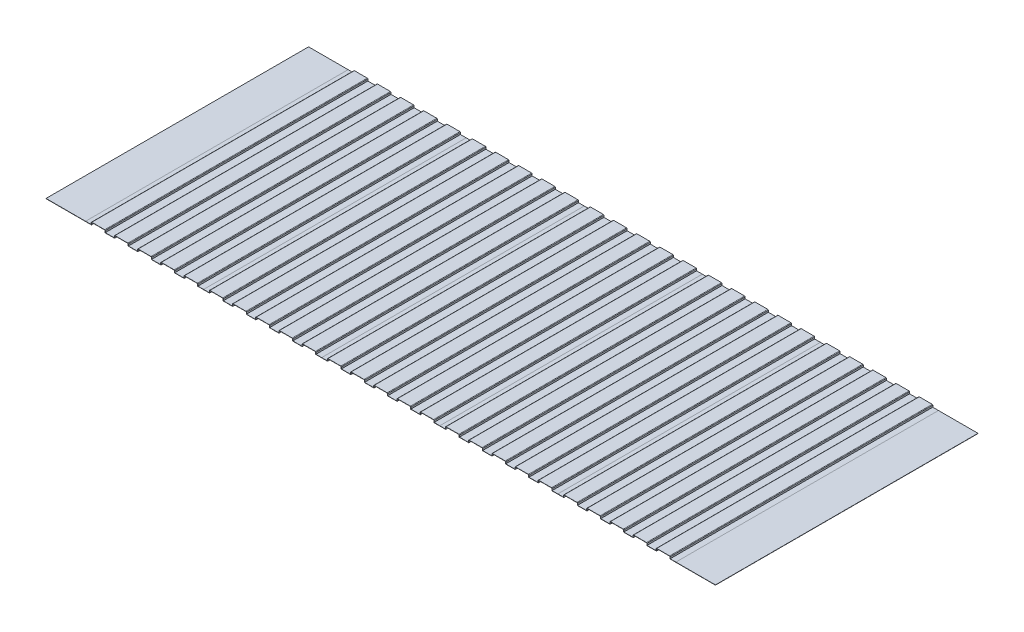
SolidWorks part; units mm, degrees
ref_plane "Front Plane" through (0, 0, 0) normal (0, 0, 1) x (1, 0, 0)
ref_plane "Top Plane" through (0, 0, 0) normal (0, 1, 0) x (1, 0, 0)
ref_plane "Right Plane" through (0, 0, 0) normal (1, 0, 0) x (0, 0, -1)
other "Configuration Table"
sketch "Sketch1" plane through (0, 0, 0) normal (0, 0, 1) x (1, 0, 0)
  line L0 (1045, 2) -> (994.5, 2)
  line L1 (994.5, 2) -> (994.5, 17)
  line L2 (989.5, 22) -> (875.5, 22)
  line L3 (870.5, 17) -> (870.5, 2)
  line L4 (870.5, 2) -> (789.5, 2)
  line L5 (789.5, 2) -> (789.5, 17)
  line L6 (784.5, 22) -> (670.5, 22)
  line L7 (665.5, 17) -> (665.5, 2)
  line L8 (665.5, 2) -> (584.5, 2)
  line L9 (584.5, 2) -> (584.5, 17)
  line L10 (579.5, 22) -> (465.5, 22)
  line L11 (460.5, 17) -> (460.5, 2)
  line L12 (460.5, 2) -> (379.5, 2)
  line L13 (379.5, 2) -> (379.5, 17)
  line L14 (374.5, 22) -> (260.5, 22)
  line L15 (255.5, 17) -> (255.5, 2)
  line L16 (255.5, 2) -> (174.5, 2)
  line L17 (174.5, 2) -> (174.5, 17)
  line L18 (169.5, 22) -> (55.5, 22)
  line L19 (50.5, 17) -> (50.5, 2)
  line L20 (50.5, 2) -> (0, 2)
  line L21 (0, 2) -> (0, 0)
  line L22 (0, 0) -> (52.5, 0)
  line L23 (52.5, 0) -> (52.5, 17)
  line L24 (55.5, 20) -> (169.5, 20)
  line L25 (172.5, 17) -> (172.5, 0)
  line L26 (172.5, 0) -> (257.5, 0)
  line L27 (257.5, 0) -> (257.5, 17)
  line L28 (260.5, 20) -> (374.5, 20)
  line L29 (377.5, 17) -> (377.5, 0)
  line L30 (377.5, 0) -> (462.5, 0)
  line L31 (462.5, 0) -> (462.5, 17)
  line L32 (465.5, 20) -> (579.5, 20)
  line L33 (582.5, 17) -> (582.5, 0)
  line L34 (582.5, 0) -> (667.5, 0)
  line L35 (667.5, 0) -> (667.5, 17)
  line L36 (670.5, 20) -> (784.5, 20)
  line L37 (787.5, 17) -> (787.5, 0)
  line L38 (787.5, 0) -> (872.5, 0)
  line L39 (872.5, 0) -> (872.5, 17)
  line L40 (875.5, 20) -> (989.5, 20)
  line L41 (992.5, 17) -> (992.5, 0)
  line L42 (992.5, 0) -> (1045, 0)
  line L43 (1045, 0) -> (1045, 2)
  arc A0 (994.5, 17) -> (989.5, 22) centre (989.5, 17) ccw
  arc A1 (875.5, 22) -> (870.5, 17) centre (875.5, 17) ccw
  arc A2 (789.5, 17) -> (784.5, 22) centre (784.5, 17) ccw
  arc A3 (670.5, 22) -> (665.5, 17) centre (670.5, 17) ccw
  arc A4 (584.5, 17) -> (579.5, 22) centre (579.5, 17) ccw
  arc A5 (465.5, 22) -> (460.5, 17) centre (465.5, 17) ccw
  arc A6 (379.5, 17) -> (374.5, 22) centre (374.5, 17) ccw
  arc A7 (260.5, 22) -> (255.5, 17) centre (260.5, 17) ccw
  arc A8 (174.5, 17) -> (169.5, 22) centre (169.5, 17) ccw
  arc A9 (55.5, 22) -> (50.5, 17) centre (55.5, 17) ccw
  arc A10 (55.5, 20) -> (52.5, 17) centre (55.5, 17) ccw
  arc A11 (172.5, 17) -> (169.5, 20) centre (169.5, 17) ccw
  arc A12 (260.5, 20) -> (257.5, 17) centre (260.5, 17) ccw
  arc A13 (377.5, 17) -> (374.5, 20) centre (374.5, 17) ccw
  arc A14 (465.5, 20) -> (462.5, 17) centre (465.5, 17) ccw
  arc A15 (582.5, 17) -> (579.5, 20) centre (579.5, 17) ccw
  arc A16 (670.5, 20) -> (667.5, 17) centre (670.5, 17) ccw
  arc A17 (787.5, 17) -> (784.5, 20) centre (784.5, 17) ccw
  arc A18 (875.5, 20) -> (872.5, 17) centre (875.5, 17) ccw
  arc A19 (992.5, 17) -> (989.5, 20) centre (989.5, 17) ccw
  dimension "D1" = 5
  dimension "D2" = 3
  dimension "D3" = 50.5
  dimension "D4" = 52.5
  dimension "D5" = 174.5
  dimension "D6" = 255.5
  dimension "D7" = 377.5
  dimension "D8" = 460.5
  dimension "D9" = 582.5
  dimension "D10" = 2
  dimension "D11" = 20
extrude "Boss-Extrude1" add sketch "Sketch1" along normal blind 2324
pattern_linear "LPattern1" count 5 spacing 1045 along (1, 0, 0) of bodies 106
sketch "Sketch2" plane through (0, 0, 0) normal (-1, 0, 0) x (0, 0, 1)
  line L4 (0, 2) -> (0, 0)
  line L5 (0, 0) -> (2324, 0)
  line L6 (2324, 0) -> (2324, 2)
  line L7 (2324, 2) -> (0, 2)
  line L8 (0, 2) -> (0, 0)
  line L9 (0, 0) -> (2324, 0)
  line L10 (2324, 0) -> (2324, 2)
  line L11 (2324, 2) -> (0, 2)
  dimension "D1" = 0
extrude "Boss-Extrude2" add sketch "Sketch2" along normal blind 350 separate body
sketch "Sketch3" plane through (5225, 0, 0) normal (1, 0, 0) x (0, 0, -1)
  line L4 (0, 0) -> (0, 2)
  line L5 (0, 2) -> (-2324, 2)
  line L6 (-2324, 2) -> (-2324, 0)
  line L7 (-2324, 0) -> (0, 0)
  line L8 (0, 0) -> (0, 2)
  line L9 (0, 2) -> (-2324, 2)
  line L10 (-2324, 2) -> (-2324, 0)
  line L11 (-2324, 0) -> (0, 0)
  dimension "D1" = 0
extrude "Boss-Extrude3" add sketch "Sketch3" along normal blind 350 separate body
